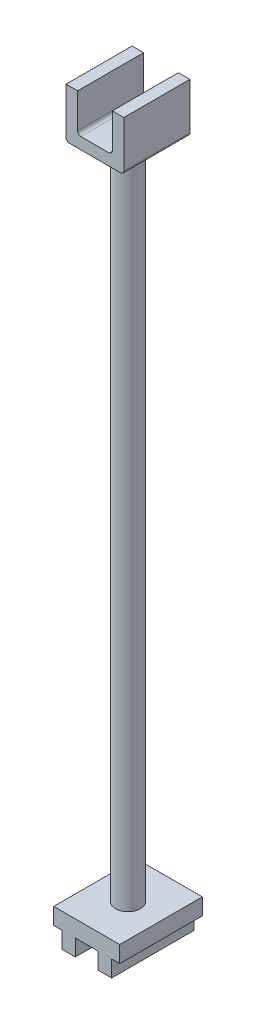
SolidWorks part; units mm, degrees
ref_plane "Front Plane" through (0, 0, 0) normal (0, 0, 1) x (1, 0, 0)
ref_plane "Top Plane" through (0, 0, 0) normal (0, 1, 0) x (1, 0, 0)
ref_plane "Right Plane" through (0, 0, 0) normal (1, 0, 0) x (0, 0, -1)
sketch "Sketch1" plane through (0, 0, 0) normal (0, 0, 1) x (1, 0, 0)
  line L0 (-10.5, 8) -> (-10.5, -8)
  line L1 (-17.5, 15) -> (-10.5, 15)
  line L2 (-17.5, 15) -> (-17.5, -15)
  line L3 (-17.5, -15) -> (17.5, -15)
  line L4 (17.5, 15) -> (17.5, -15)
  line L5 (-17.5, 15) -> (17.5, -15) construction
  line L6 (-17.5, -15) -> (17.5, 15) construction
  line L7 (-10.5, -8) -> (10.5, -8)
  line L8 (10.5, 8) -> (10.5, -8)
  line L10 (-10.5, 8) -> (-10.5, 15)
  line L11 (10.5, 8) -> (10.5, 15)
  line L12 (10.5, 15) -> (17.5, 15)
  line L13 (-17.5, 15) -> (17.5, 15) construction
  line L14 (-10.5, 8) -> (10.5, 8) construction
  point P0 (0, 0)
  dimension "D1" = 35
  dimension "D2" = 30
  dimension "D3" = 7
extrude "Boss-Extrude1" add sketch "Sketch1" along normal mid plane 40
fillet "Fillet1" radius 2 4 edges at (17.5, -15, 0) (-17.5, -15, 0) (10.5, -8, 0) (-10.5, -8, 0)
sketch "Sketch2" plane through (0, -15, 0) normal (0, -1, 0) x (1, 0, 0)
  circle A0 centre (0, 0) radius 7.5
  dimension "D1" = 15
extrude "Boss-Extrude2" add sketch "Sketch2" along normal blind 400
sketch "Sketch3" plane through (0, -415, 0) normal (0, -1, 0) x (1, 0, 0)
  line L1 (-20, 25) -> (20, 25)
  line L2 (-20, 25) -> (-20, -25)
  line L3 (-20, -25) -> (20, -25)
  line L4 (20, 25) -> (20, -25)
  line L5 (-20, 25) -> (20, -25) construction
  line L6 (-20, -25) -> (20, 25) construction
  point P0 (0, 0)
  dimension "D1" = 50
  dimension "D2" = 40
extrude "Boss-Extrude3" add sketch "Sketch3" along normal blind 10
sketch "Sketch4" plane through (0, -425, 0) normal (0, -1, 0) x (1, 0, 0)
  line L0 (20, 25) -> (-20, 25) construction
  line L1 (-15.1, 25) -> (-6.9, 25)
  line L2 (-15.1, 25) -> (-15.1, -25)
  line L3 (-15.1, -25) -> (-6.9, -25)
  line L4 (-6.9, 25) -> (-6.9, -25)
  line L5 (-15.1, 25) -> (-6.9, -25) construction
  line L6 (-15.1, -25) -> (-6.9, 25) construction
  line L7 (0, 0) -> (0, 11.8275) construction
  line L8 (15.1, -25) -> (6.9, 25) construction
  line L9 (15.1, 25) -> (6.9, -25) construction
  line L10 (6.9, 25) -> (6.9, -25)
  line L11 (15.1, -25) -> (6.9, -25)
  line L12 (15.1, 25) -> (15.1, -25)
  line L13 (15.1, 25) -> (6.9, 25)
  point P0 (-11, 0)
  point P14 (11, 0)
  dimension "D1" = 11
  dimension "D2" = 8.2
extrude "Boss-Extrude4" add sketch "Sketch4" along normal blind 10
